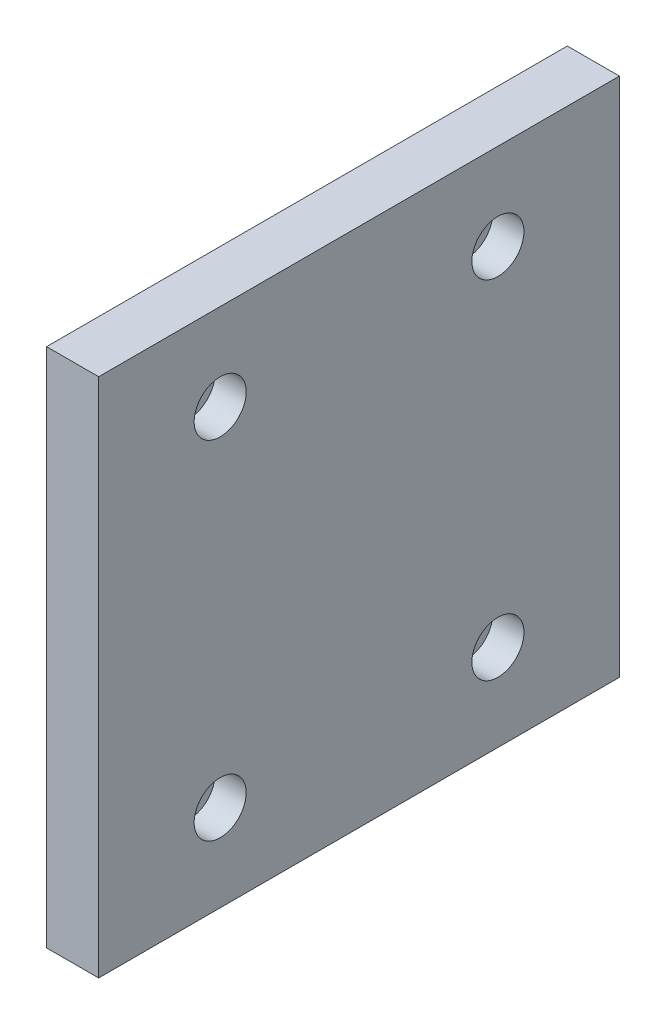
from build123d import *

# Parameters (mm, degrees)
SKETCH_1_W                = 150
SKETCH_1_H                = 150
EXTRUDE_1_DEPTH           = 15
HOLE_WIZARD_1_D           = 9
HOLE_WIZARD_1_CBORE_D     = 15
HOLE_WIZARD_1_CBORE_DEPTH = 9


with BuildPart() as part:
    # 草图1 → 凸台-拉伸1 (new body)
    with BuildSketch(Plane(origin=(0, 0, 0), x_dir=(0, 0, -1), z_dir=(1, 0, 0))):
        Rectangle(SKETCH_1_W, SKETCH_1_H)
    extrude(amount=EXTRUDE_1_DEPTH)

    # 打孔尺寸(%根据)内六角圆柱头螺钉的类型1 (through all)
    with Locations(Plane(origin=(15, 0, 0), x_dir=(0, 0, -1), z_dir=(1, 0, 0))):
        with Locations((-40, 50), (40, 50), (-40, -50), (40, -50)):
            CounterBoreHole(HOLE_WIZARD_1_D / 2, HOLE_WIZARD_1_CBORE_D / 2, HOLE_WIZARD_1_CBORE_DEPTH)


solid = part.part
